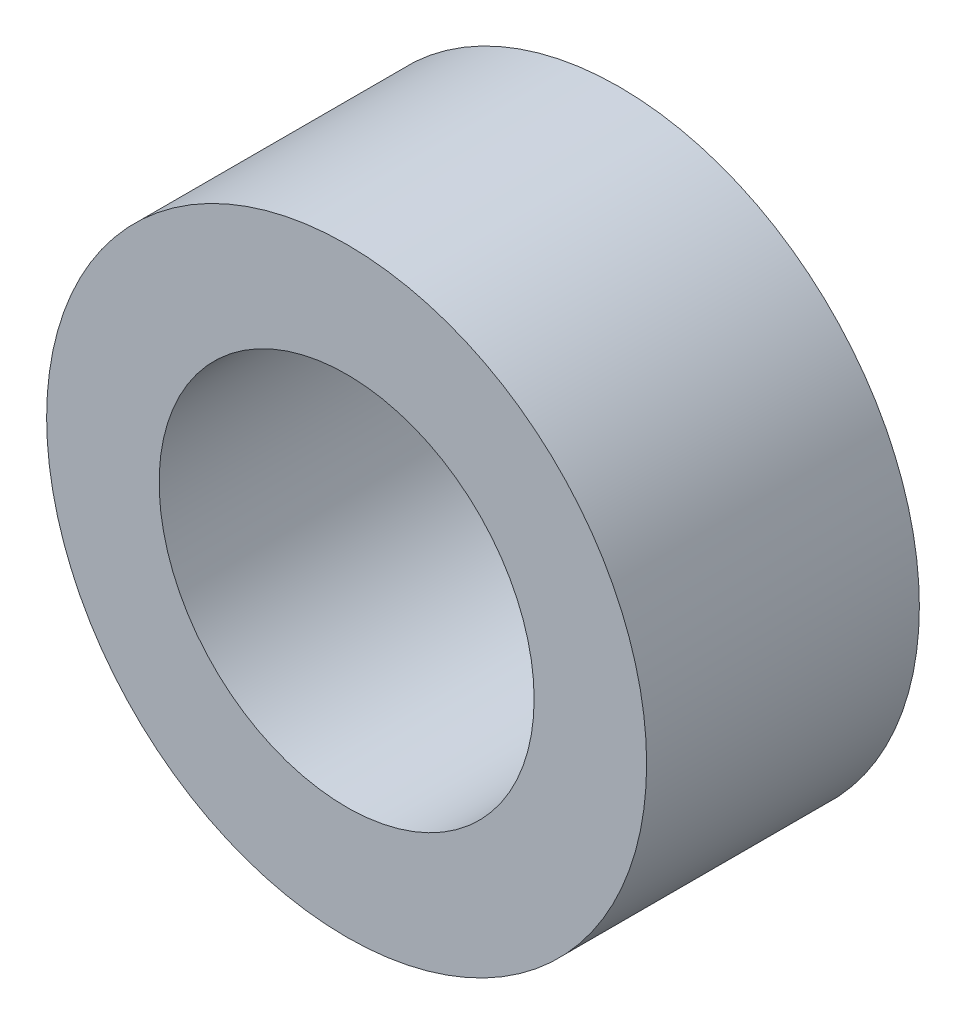
from build123d import *

# Parameters (mm, degrees)
SKETCH1_R           = 4.4
SKETCH1_R_2         = 2.75
BOSS_EXTRUDE1_DEPTH = 4


with BuildPart() as part:
    # Sketch1 → Boss-Extrude1 (new body)
    with BuildSketch(Plane.XY):
        Circle(SKETCH1_R)
        Circle(SKETCH1_R_2, mode=Mode.SUBTRACT)
    extrude(amount=BOSS_EXTRUDE1_DEPTH)


solid = part.part
